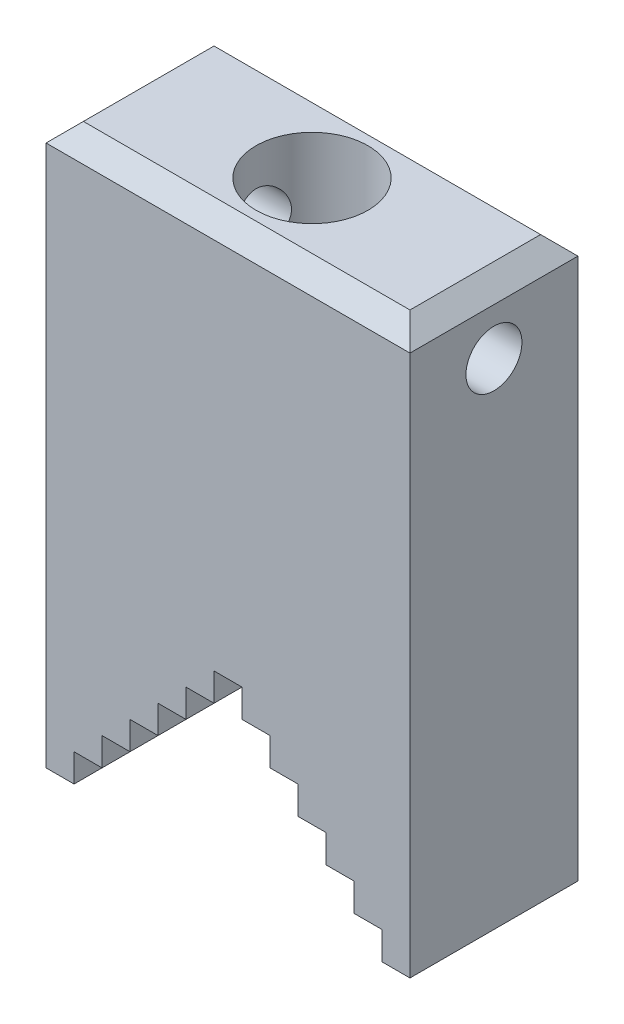
from build123d import *

# Parameters (mm, degrees)
BOSS_EXTRUDE1_DEPTH = 9
CHAMFER1_SIZE       = 2
SKETCH2_R           = 3
CUT_EXTRUDE1_DEPTH  = 51.019996002


with BuildPart() as part:
    # Sketch1 → Boss-Extrude1 (new, symmetric)
    with BuildSketch(Plane.XY):
        Polygon((-16.5, -30), (-16.5, -27), (-13.5, -27), (-13.5, -24), (-10.5, -24), (-10.5, -21), (-7.5, -21), (-7.5, -18), (-4.5, -18), (-4.5, -15), (-1.5, -15), (-1.5, -12), (1.5, -12), (1.5, -15), (4.5, -15), (4.5, -18), (7.5, -18), (7.5, -21), (10.5, -21), (10.5, -24), (13.5, -24), (13.5, -27), (16.5, -27), (16.5, -30), (19.5, -30), (19.5, 30), (-19.5, 30), (-19.5, -30), align=None)
    extrude(amount=BOSS_EXTRUDE1_DEPTH, both=True)

    # Chamfer1
    chamfer1_edges = [part.edges().sort_by_distance(p)[0] for p in [
        (0, 30, 9),
        (0, 30, -9),
        (-19.5, 30, 0),
        (19.5, 30, 0),
    ]]
    chamfer(chamfer1_edges, length=CHAMFER1_SIZE)

    # Sketch2 → Cut-Extrude1 (cut, through all)
    with BuildSketch(Plane(origin=(19.5, 0, 0), x_dir=(0, 0, -1), z_dir=(1, 0, 0))):
        with Locations(Location((0, 23, 0), (0, 0, 90))):
            Circle(SKETCH2_R)
    extrude(amount=-CUT_EXTRUDE1_DEPTH, mode=Mode.SUBTRACT)

    # Sketch3 → Cut-Revolve1 (revolve, cut)
    with BuildSketch(Plane.XY, mode=Mode.PRIVATE) as cut_revolve1_sk:
        Polygon((0, 30), (6, 30), (6, 10), (0, 6.535898385), align=None)
    revolve(cut_revolve1_sk.sketch.rotate(Axis((0, 31.728134739, 0), (0, -1, 0)), 90), axis=Axis((0, 31.728134739, 0), (0, -1, 0)), mode=Mode.SUBTRACT)


solid = part.part
